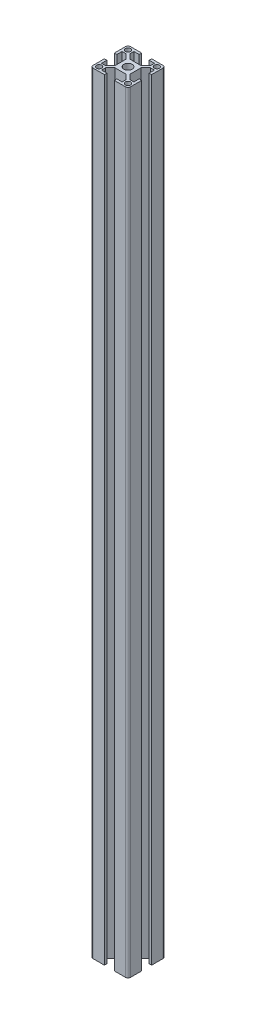
SolidWorks part; units mm, degrees
ref_plane "前视基准面" through (0, 0, 0) normal (0, 0, 1) x (1, 0, 0)
ref_plane "上视基准面" through (0, 0, 0) normal (0, 1, 0) x (1, 0, 0)
ref_plane "右视基准面" through (0, 0, 0) normal (1, 0, 0) x (0, 0, -1)
sketch "草图1" plane through (0, 0, 0) normal (0, 1, 0) x (1, 0, 0)
  line L44 (6.75, -28) -> (11, -28)
  line L45 (11, -28) -> (11, -30)
  line L46 (11, -30) -> (2, -30)
  line L47 (0, -28) -> (0, -19)
  line L48 (0, -19) -> (2, -19)
  line L49 (2, -19) -> (2, -23.25)
  line L50 (28, -30) -> (19, -30)
  line L51 (19, -30) -> (19, -28)
  line L52 (23.25, -28) -> (23.25, -24.6642)
  line L53 (19, -28) -> (23.25, -28)
  line L54 (30, -19) -> (30, -28)
  line L55 (28, -19) -> (30, -19)
  line L56 (28, -23.25) -> (28, -19)
  line L57 (24.6642, -23.25) -> (28, -23.25)
  line L58 (21, -19.5858) -> (24.6642, -23.25)
  line L59 (23.25, -24.6642) -> (19.5858, -21)
  line L60 (6.75, -24.6642) -> (6.75, -28)
  line L61 (2, -23.25) -> (5.3358, -23.25)
  line L62 (5.3358, -23.25) -> (9, -19.5858)
  line L63 (10.4142, -21) -> (6.75, -24.6642)
  line L64 (19.5858, -21) -> (10.4142, -21)
  line L65 (9, -19.5858) -> (9, -10.4142)
  line L66 (21, -10.4142) -> (21, -19.5858)
  line L67 (30, -11) -> (28, -11)
  line L68 (28, -11) -> (28, -6.75)
  line L69 (28, -6.75) -> (24.6642, -6.75)
  line L70 (24.6642, -6.75) -> (21, -10.4142)
  line L71 (19.5858, -9) -> (23.25, -5.3358)
  line L72 (10.4142, -9) -> (19.5858, -9)
  line L73 (6.75, -5.3358) -> (10.4142, -9)
  line L74 (9, -10.4142) -> (5.3358, -6.75)
  line L75 (2, -11) -> (0, -11)
  line L76 (2, -6.75) -> (2, -11)
  line L77 (5.3358, -6.75) -> (2, -6.75)
  line L78 (6.75, -2) -> (6.75, -5.3358)
  line L79 (23.25, -5.3358) -> (23.25, -2)
  line L80 (23.25, -2) -> (19, -2)
  line L81 (19, -2) -> (19, 0)
  line L82 (11, 0) -> (11, -2)
  line L83 (11, -2) -> (6.75, -2)
  line L84 (30, -2) -> (30, -11)
  line L85 (19, 0) -> (28, 0)
  line L86 (2, 0) -> (11, 0)
  line L87 (0, -11) -> (0, -2)
  line L88 (0, -15) -> (30, -15) construction
  line L89 (15, -30) -> (15, 0) construction
  line L90 (0, 0) -> (30, -30) construction
  line L91 (0, -30) -> (30, 0) construction
  arc A9 (0, -28) -> (2, -30) centre (2, -28) ccw
  circle A10 centre (3.375, -26.625) radius 2.1
  circle A11 centre (26.625, -26.625) radius 2.1
  arc A12 (28, -30) -> (30, -28) centre (28, -28) ccw
  circle A13 centre (15, -15) radius 3.4
  circle A14 centre (3.375, -3.375) radius 2.1
  circle A15 centre (26.625, -3.375) radius 2.1
  arc A16 (30, -2) -> (28, 0) centre (28, -2) ccw
  arc A17 (2, 0) -> (0, -2) centre (2, -2) ccw
  dimension "D2" = 15
  dimension "D5" = 6.8
  dimension "D8" = 6
  dimension "D11" = 23.25
  dimension "D12" = 3.375
  dimension "D13" = 23.25
  dimension "D14" = 4.2
  dimension "D15" = 2
  dimension "D16" = 2
  dimension "D23" = 2
  dimension "D24" = 2
  dimension "D1" = 15
  dimension "D3" = 45
  dimension "D4" = 45
  dimension "D6" = 30
  dimension "D7" = 30
  dimension "D9" = 12
  dimension "D10" = 3.375
  dimension "D17" = 11
  dimension "D18" = 8
  dimension "D19" = 2
  dimension "D20" = 2
  dimension "D21" = 11
  dimension "D22" = 8
  dimension "D25" = 2
  dimension "D26" = 2
  dimension "D27" = 6.75
  dimension "D28" = 16.5
  dimension "D29" = 6.75
  dimension "D30" = 16.5
  dimension "D31" = 12
  dimension "D32" = 6
  dimension "D33" = 2
  dimension "D34" = 1
  dimension "D35" = 2
  dimension "D36" = 1
extrude "拉伸1" add sketch "草图1" along normal blind 620
